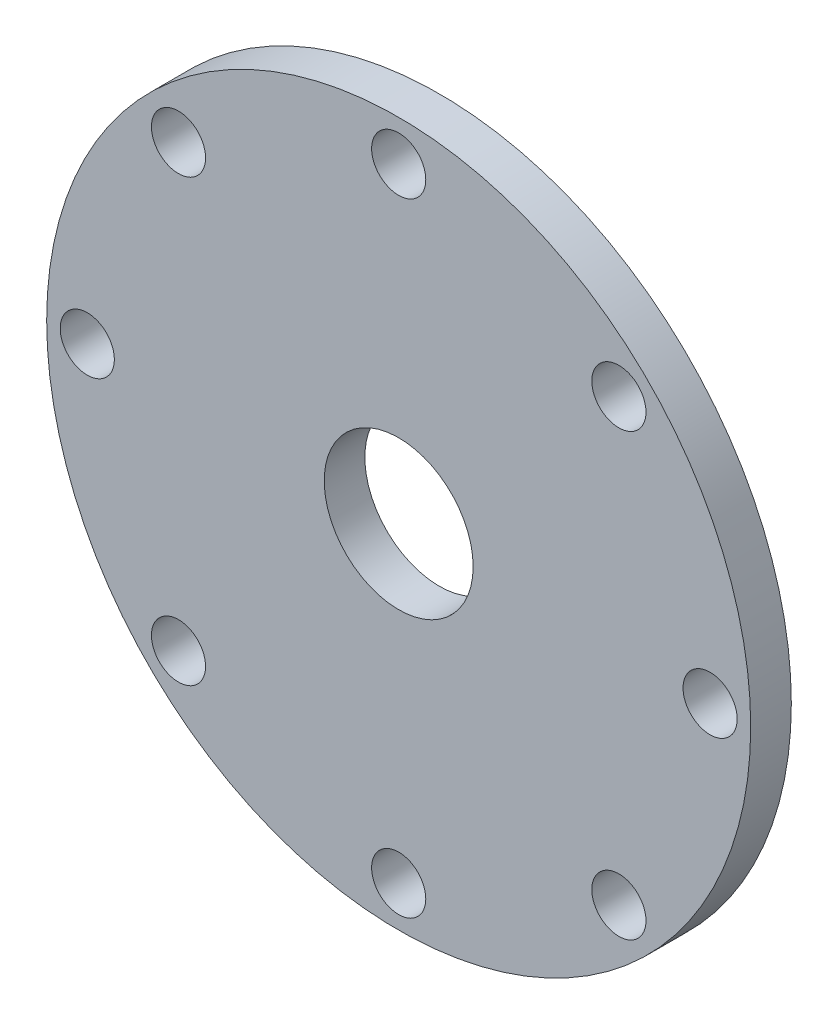
SolidWorks part; units mm, degrees
ref_plane "Front Plane" through (0, 0, 0) normal (0, 0, 1) x (1, 0, 0)
ref_plane "Top Plane" through (0, 0, 0) normal (0, 1, 0) x (1, 0, 0)
ref_plane "Right Plane" through (0, 0, 0) normal (1, 0, 0) x (0, 0, -1)
other "Configuration Table"
sketch "Sketch2" plane through (0, 0, 0) normal (0, 0, 1) x (1, 0, 0)
  circle A1 centre (0, 0) radius 27.5
  circle A3 centre (0, 0) radius 130
  dimension "D1" = 55
extrude "Boss-Extrude1" add sketch "Sketch2" along normal blind 15
sketch "Sketch3" plane through (0, 0, 0) normal (0, 0, 1) x (1, 0, 0)
  circle A0 centre (-115, 0) radius 10
  dimension "D1" = 20
extrude "Cut-Extrude1" cut sketch "Sketch3" against normal through all both and the other way through all
pattern_circular "CirPattern1" count 8 over 360 about axis through (0, 0, 0) along (0, 0, 1) of "Cut-Extrude1"
